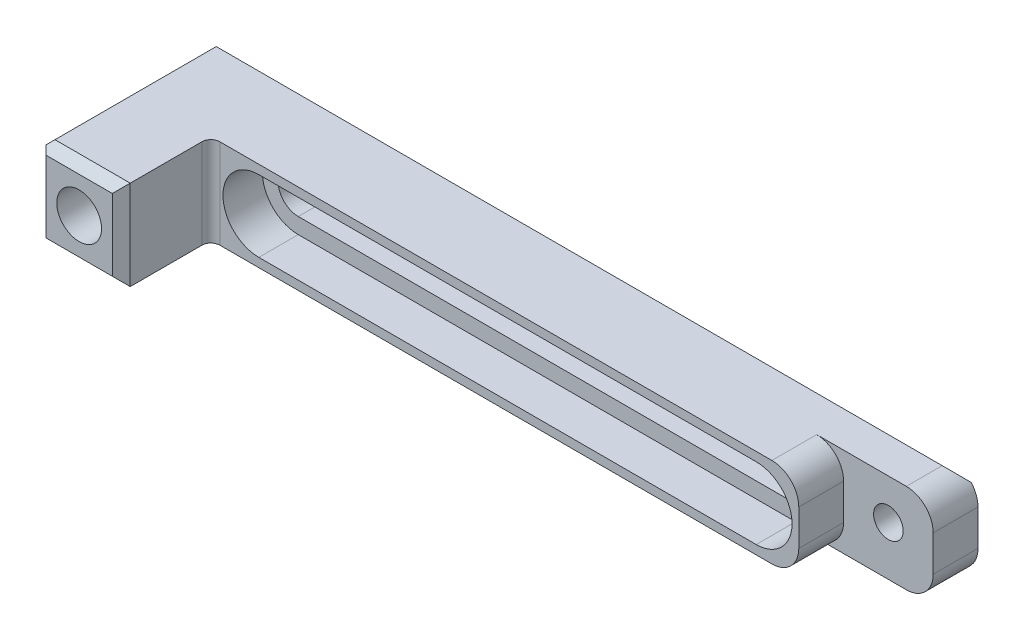
from build123d import *

# Parameters (mm, degrees)
SKETCH1_W             = 85
SKETCH1_H             = 10
BOSS_EXTRUDE1_DEPTH   = 10
CUT_EXTRUDE1_DEPTH    = 4.4
CUT_EXTRUDE2_DEPTH    = 45.018291652
SKETCH4_W             = 9.4
SKETCH4_H             = 10
BOSS_EXTRUDE2_DEPTH   = 10
SKETCH5_W             = 10
SKETCH5_H             = 10
CUT_EXTRUDE3_DEPTH    = 5
M6_TAPPED_HOLE1_D     = 5
M6_TAPPED_HOLE1_DEPTH = 17
M6_TAPPED_HOLE1_TIP   = 1.502151548
M4_TAPPED_HOLE1_D     = 3.3
M4_TAPPED_HOLE1_DEPTH = 11.5
M4_TAPPED_HOLE1_TIP   = 0.991420021
FILLET1_R             = 3
CHAMFER2_SIZE         = 1
FILLET2_R             = 1
CHAMFER3_SIZE         = 1
FILLET3_R             = 3


with BuildPart() as part:
    # Sketch1 → Boss-Extrude1 (new body)
    with BuildSketch(Plane(origin=(0, 0, 0), x_dir=(1, 0, 0), z_dir=(0, 1, 0))):
        Rectangle(SKETCH1_W, SKETCH1_H)
    extrude(amount=BOSS_EXTRUDE1_DEPTH)

    # Sketch2 → Cut-Extrude1 (cut)
    with BuildSketch(Plane.XY.offset(5)):
        with BuildLine():
            Line((-27.75, 9), (27.75, 9))
            ThreePointArc((27.75, 9), (31.75, 5), (27.75, 1))
            Line((27.75, 1), (-27.75, 1))
            ThreePointArc((-27.75, 1), (-31.75, 5), (-27.75, 9))
        make_face()
    extrude(amount=-CUT_EXTRUDE1_DEPTH, mode=Mode.SUBTRACT)

    # Sketch3 → Cut-Extrude2 (cut, through all)
    with BuildSketch(Plane.XY.offset(0.6)):
        with BuildLine():
            Line((-27.75, 7.25), (27.75, 7.25))
            ThreePointArc((27.75, 7.25), (30, 5), (27.75, 2.75))
            Line((27.75, 2.75), (-27.75, 2.75))
            ThreePointArc((-27.75, 2.75), (-30, 5), (-27.75, 7.25))
        make_face()
    extrude(amount=-CUT_EXTRUDE2_DEPTH, mode=Mode.SUBTRACT)

    # Sketch4 → Boss-Extrude2 (add)
    with BuildSketch(Plane.XY.offset(5)):
        with Locations((-37.8, 5)):
            Rectangle(SKETCH4_W, SKETCH4_H)
    extrude(amount=BOSS_EXTRUDE2_DEPTH)

    # Sketch5 → Cut-Extrude3 (cut)
    with BuildSketch(Plane.XY.offset(5)):
        with Locations((37.5, 5)):
            Rectangle(SKETCH5_W, SKETCH5_H)
    extrude(amount=-CUT_EXTRUDE3_DEPTH, mode=Mode.SUBTRACT)

    # M6 Tapped Hole1
    with Locations(Plane.XY.offset(15)):
        with Locations((-37.8, 5)):
            Hole(M6_TAPPED_HOLE1_D / 2, depth=M6_TAPPED_HOLE1_DEPTH)
            with Locations((0, 0, -(M6_TAPPED_HOLE1_DEPTH + M6_TAPPED_HOLE1_TIP / 2))):  # 118° drill point
                Cone(0, M6_TAPPED_HOLE1_D / 2, M6_TAPPED_HOLE1_TIP, mode=Mode.SUBTRACT)

    # M4 Tapped Hole1
    with Locations(Plane.XY):
        with Locations((37.5, 5.5)):
            Hole(M4_TAPPED_HOLE1_D / 2, depth=M4_TAPPED_HOLE1_DEPTH)
            with Locations((0, 0, -(M4_TAPPED_HOLE1_DEPTH + M4_TAPPED_HOLE1_TIP / 2))):  # 118° drill point
                Cone(0, M4_TAPPED_HOLE1_D / 2, M4_TAPPED_HOLE1_TIP, mode=Mode.SUBTRACT)

    # Fillet1
    fillet1_edges = [part.edges().sort_by_distance(p)[0] for p in [
        (32.5, 0, 2.5),
        (32.5, 10, 2.5),
    ]]
    fillet(fillet1_edges, radius=FILLET1_R)

    # Chamfer2
    chamfer2_edges = [part.edges().sort_by_distance(p)[0] for p in [
        (-37.8, 10, 15),
        (-33.1, 5, 15),
        (-42.5, 5, 15),
        (-37.8, 0, 15),
    ]]
    chamfer(chamfer2_edges, length=CHAMFER2_SIZE)

    # Fillet2
    fillet2_edges = [part.edges().sort_by_distance(p)[0] for p in [
        (-33.1, 5, 5),
    ]]
    fillet(fillet2_edges, radius=FILLET2_R)

    # Chamfer3
    chamfer3_edges = [part.edges().sort_by_distance(p)[0] for p in [
        (0, 10, -5),
        (-42.5, 10, 4.5),
        (0, 0, -5),
        (-42.5, 0, 4.5),
        (-42.5, 5, -5),
    ]]
    chamfer(chamfer3_edges, length=CHAMFER3_SIZE)

    # Fillet3
    fillet3_edges = [part.edges().sort_by_distance(p)[0] for p in [
        (42.5, 0, -2),
        (42.5, 10, -2),
    ]]
    fillet(fillet3_edges, radius=FILLET3_R)


solid = part.part
